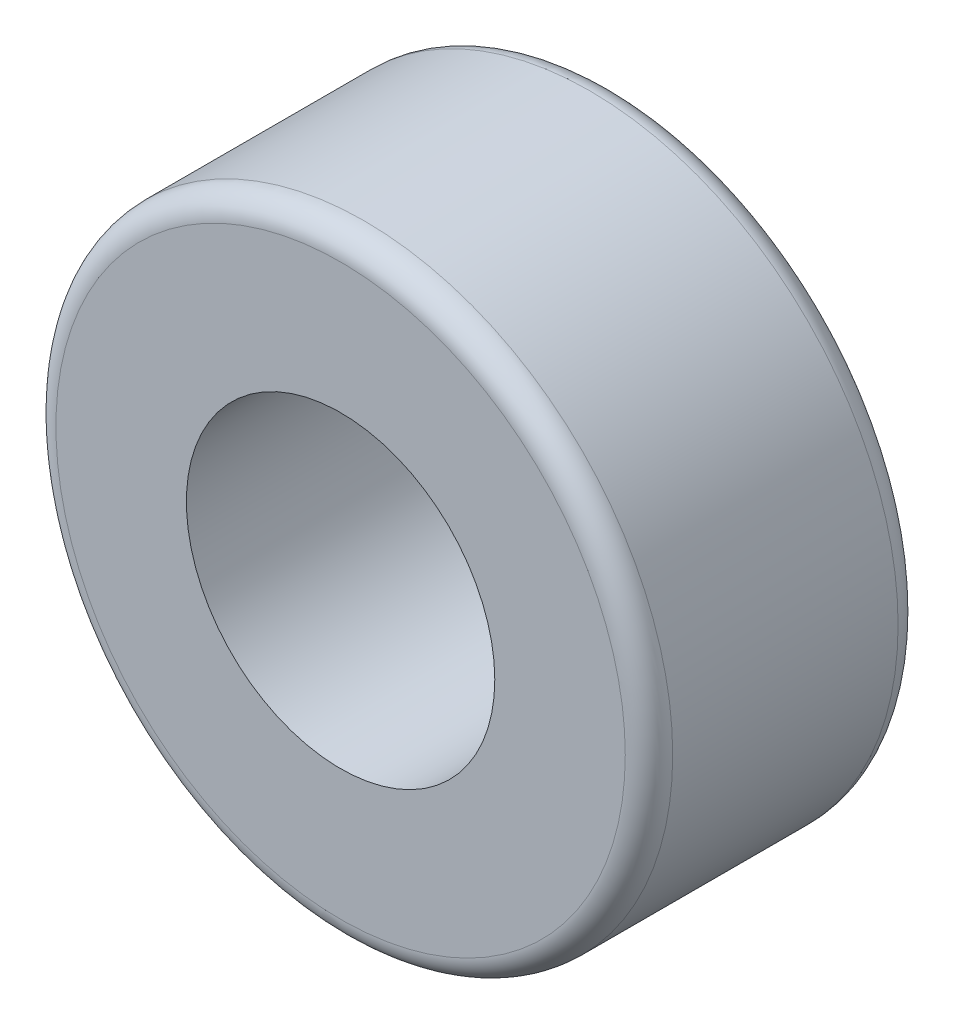
SolidWorks part; units mm, degrees
ref_plane "前视基准面" through (0, 0, 0) normal (0, 0, 1) x (1, 0, 0)
ref_plane "上视基准面" through (0, 0, 0) normal (0, 1, 0) x (1, 0, 0)
ref_plane "右视基准面" through (0, 0, 0) normal (1, 0, 0) x (0, 0, -1)
sketch "草图1" plane through (0, 0, 0) normal (0, 0, 1) x (1, 0, 0)
  circle A0 centre (0, 0) radius 13
  circle A1 centre (0, 0) radius 6.5
  dimension "D1" = 26
  dimension "D2" = 13
extrude "凸台-拉伸1" add sketch "草图1" along normal blind 11.5
fillet "圆角1" radius 1 2 edges at (13, 0, 0) (13, 0, 11.5)
